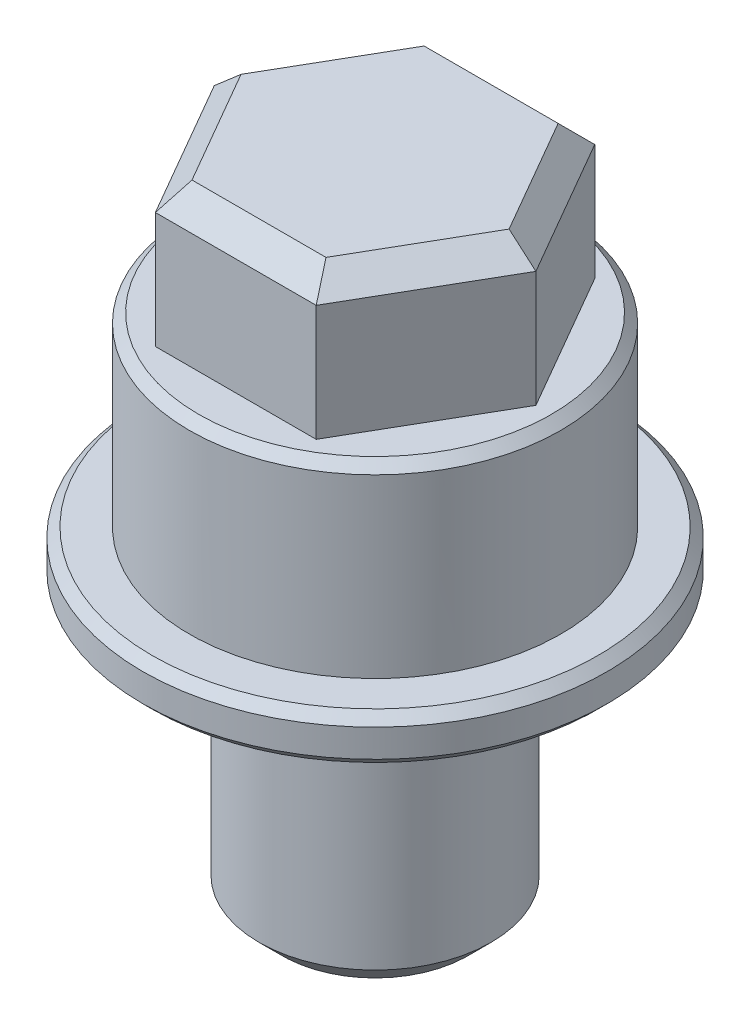
from build123d import *

# Parameters (mm, degrees)
SKETCH4_OUTSIDE_W  = 15.98
SKETCH4_OUTSIDE_H  = 15.98
CUT_EXTRUDE2_DEPTH = 3
CHAMFER1_SIZE      = 0.5
CHAMFER2_SIZE      = 0.2


with BuildPart() as part:
    # Sketch2 → Revolve1 (revolve)
    with BuildSketch(Plane.XY, mode=Mode.PRIVATE) as revolve1_sk:
        Polygon((0, 0), (2.5, 0), (2.5, 6), (5, 6), (5, 7), (4, 7), (4, 14), (0, 14), align=None)
    revolve(revolve1_sk.sketch.rotate(Axis((0, 0, 0), (0, 1, 0)), 90), axis=Axis((0, 0, 0), (0, 1, 0)))

    # Sketch4 outside → Cut-Extrude2 (cut)
    with BuildSketch(Plane(origin=(0, 14, 0), x_dir=(1, 0, 0), z_dir=(0, 1, 0))):
        Rectangle(SKETCH4_OUTSIDE_W, SKETCH4_OUTSIDE_H)
        Polygon((1.732050808, 3), (-1.732050808, 3), (-3.464101615, 0), (-1.732050808, -3), (1.732050808, -3), (3.464101615, 0), align=None, mode=Mode.SUBTRACT)
    extrude(amount=-CUT_EXTRUDE2_DEPTH, mode=Mode.SUBTRACT)

    # Chamfer1
    chamfer1_edges = [part.edges().sort_by_distance(p)[0] for p in [
        (2.598076211, 14, -1.5),
        (2.598076211, 14, 1.5),
        (0, 14, 3),
        (-2.598076211, 14, 1.5),
        (-2.598076211, 14, -1.5),
        (0, 14, -3),
        (0, 0, 2.5),
    ]]
    chamfer(chamfer1_edges, length=CHAMFER1_SIZE)

    # Chamfer2
    chamfer2_edges = [part.edges().sort_by_distance(p)[0] for p in [
        (0, 11, 4),
        (0, 7, 5),
        (0, 6, 5),
    ]]
    chamfer(chamfer2_edges, length=CHAMFER2_SIZE)


solid = part.part
